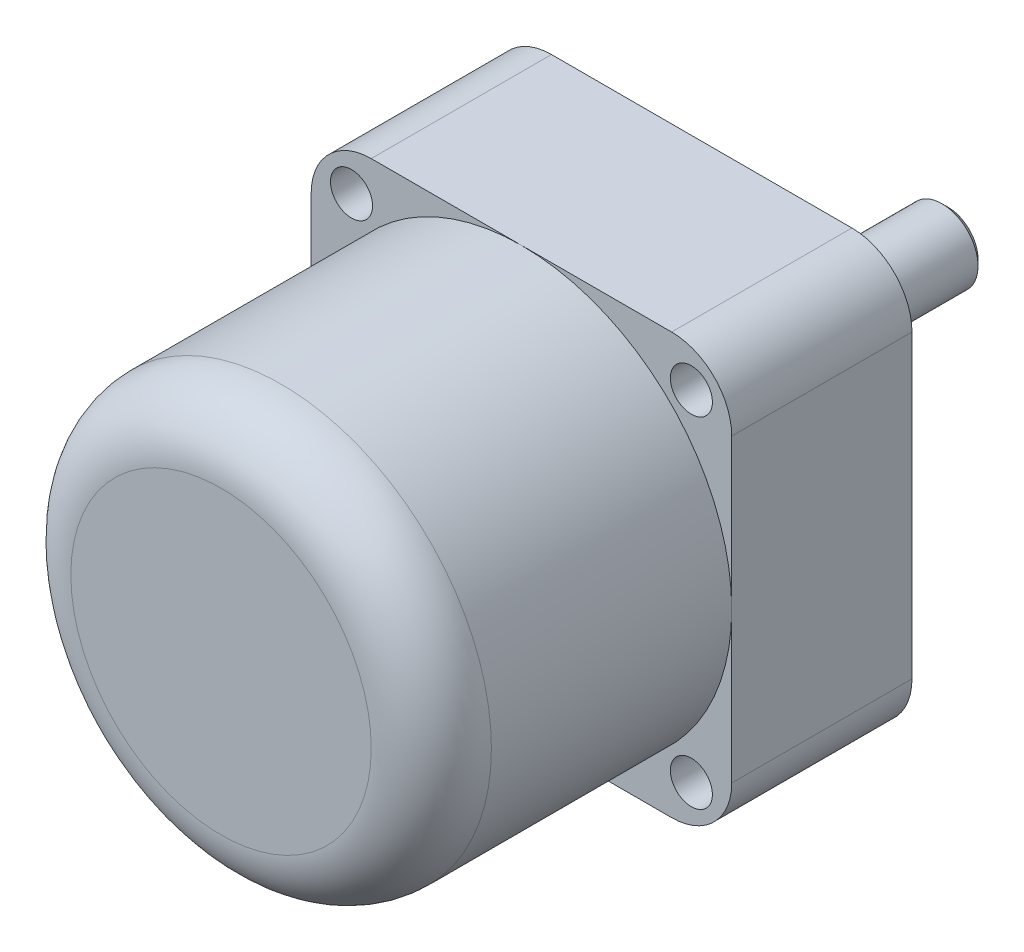
from build123d import *

# Parameters (mm, degrees)
SKETCH1_W           = 70
SKETCH1_H           = 70
BOSS_EXTRUDE1_DEPTH = 30
FILLET2_R           = 10
SKETCH3_R           = 3.5
CUT_EXTRUDE1_DEPTH  = 60
SKETCH4_R           = 22.5
BOSS_EXTRUDE3_DEPTH = 6
SKETCH5_R           = 6
BOSS_EXTRUDE4_DEPTH = 35
CHAMFER1_SIZE       = 1
CHAMFER2_SIZE       = 1
CIRPATTERN1_COUNT   = 4
SKETCH6_R           = 35
BOSS_EXTRUDE5_DEPTH = 50
FILLET3_R           = 10


with BuildPart() as part:
    # Sketch1 → Boss-Extrude1 (new body)
    with BuildSketch(Plane.XY):
        Rectangle(SKETCH1_W, SKETCH1_H)
    extrude(amount=BOSS_EXTRUDE1_DEPTH)

    # Fillet2
    fillet2_edges = [part.edges().sort_by_distance(p)[0] for p in [
        (-35, 35, 15),
        (35, 35, 15),
        (35, -35, 15),
        (-35, -35, 15),
    ]]
    fillet(fillet2_edges, radius=FILLET2_R)

    # Sketch3 → Cut-Extrude1 (cut)
    with BuildSketch(Plane.XY.offset(30)):
        with Locations((-28.284271247, 28.284271247)):
            Circle(SKETCH3_R)
    cut_extrude1 = extrude(amount=-CUT_EXTRUDE1_DEPTH, mode=Mode.SUBTRACT)

    # Sketch4 → Boss-Extrude3 (add)
    with BuildSketch(Plane(origin=(0, 0, 0), x_dir=(-1, 0, 0), z_dir=(0, 0, -1))):
        with Locations(Location((0, 0, 0), (0, 0, 180))):
            Circle(SKETCH4_R)
    extrude(amount=BOSS_EXTRUDE3_DEPTH)

    # Sketch5 → Boss-Extrude4 (add)
    with BuildSketch(Plane(origin=(0, 0, -6), x_dir=(-1, 0, 0), z_dir=(0, 0, -1))):
        Circle(SKETCH5_R)
    extrude(amount=BOSS_EXTRUDE4_DEPTH)

    # Chamfer1
    chamfer1_edges = [part.edges().sort_by_distance(p)[0] for p in [
        (6, 0, -41),
    ]]
    chamfer(chamfer1_edges, length=CHAMFER1_SIZE)

    # Chamfer2
    chamfer2_edges = [part.edges().sort_by_distance(p)[0] for p in [
        (-22.5, 0, -6),
    ]]
    chamfer(chamfer2_edges, length=CHAMFER2_SIZE)

    # CirPattern1: Cut-Extrude1 ×4 about axis
    cirpattern1_axis = Axis((0, 0, 0), (0, 0, 1))
    for i in range(1, CIRPATTERN1_COUNT):
        add(cut_extrude1.rotate(cirpattern1_axis, i * 360 / CIRPATTERN1_COUNT), mode=Mode.SUBTRACT)

    # Sketch6 → Boss-Extrude5 (add)
    with BuildSketch(Plane.XY.offset(30)):
        Circle(SKETCH6_R)
    extrude(amount=BOSS_EXTRUDE5_DEPTH)

    # Fillet3
    fillet3_edges = [part.edges().sort_by_distance(p)[0] for p in [
        (-35, 0, 80),
    ]]
    fillet(fillet3_edges, radius=FILLET3_R)


solid = part.part
